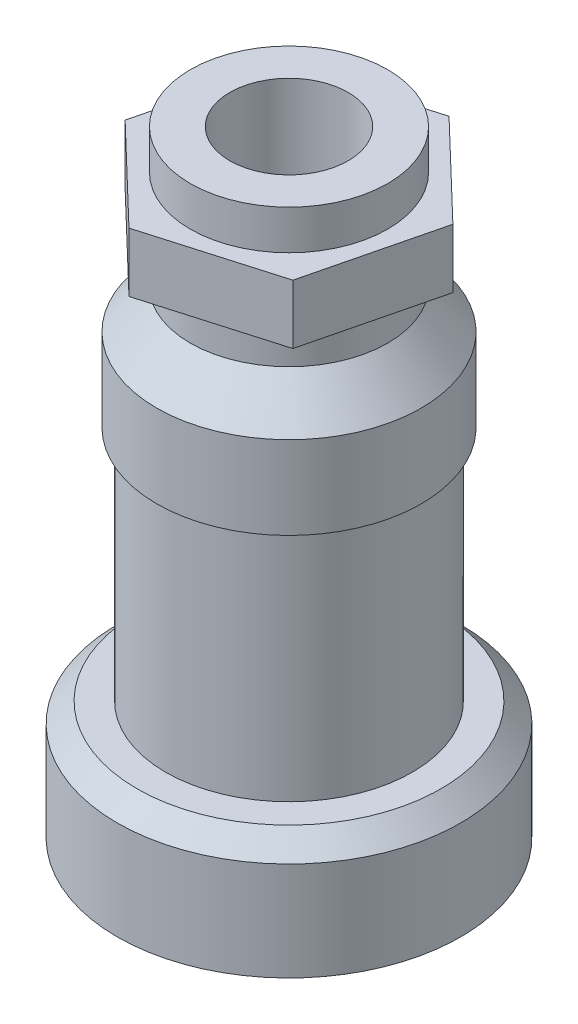
SolidWorks part; units mm, degrees
ref_plane "Front Plane" through (0, 0, 0) normal (0, 0, 1) x (1, 0, 0)
ref_plane "Top Plane" through (0, 0, 0) normal (0, 1, 0) x (1, 0, 0)
ref_plane "Right Plane" through (0, 0, 0) normal (1, 0, 0) x (0, 0, -1)
sketch "Sketch1" plane through (0, 0, 0) normal (0, 0, 1) x (1, 0, 0)
  line L0 (0, 0) -> (0, -35.4245) construction
  line L1 (0, 0) -> (5, 0)
  line L2 (5, 0) -> (5, -7)
  line L4 (5, -7) -> (6.7, -9)
  line L5 (6.7, -9) -> (6.7, -13.2)
  line L6 (6.7, -13.2) -> (6.25, -13.2)
  line L7 (6.25, -13.2) -> (6.25, -25.2)
  line L8 (6.25, -25.2) -> (8.7, -25.2)
  line L9 (8.7, -25.2) -> (8.7, -31.2)
  line L10 (8.7, -31.2) -> (0, -31.2)
  line L11 (0, -31.2) -> (0, 0)
  dimension "D1" = 5
  dimension "D2" = 7
  dimension "D3" = 6.7
  dimension "D4" = 2
  dimension "D5" = 4.2
  dimension "D6" = 6.25
  dimension "D7" = 12
  dimension "D8" = 8.7
  dimension "D9" = 6
revolve "Revolve1" add sketch "Sketch1" angle 360 about L0
ref_plane "Plane1" through (0, -2, 0) normal (0, 1, 0) x (1, 0, 0)
sketch "Sketch2" plane through (0, -2, 0) normal (0, 1, 0) x (1, 0, 0)
  line L1 (-1.6001, -6.5061) -> (4.8344, -4.6388)
  line L2 (4.8344, -4.6388) -> (6.4345, 1.8674)
  line L3 (6.4345, 1.8674) -> (1.6001, 6.5061)
  line L4 (1.6001, 6.5061) -> (-4.8344, 4.6388)
  line L5 (-4.8344, 4.6388) -> (-6.4345, -1.8674)
  line L6 (-6.4345, -1.8674) -> (-1.6001, -6.5061)
  circle A0 centre (0, 0) radius 5.8024 construction
extrude "Boss-Extrude1" add sketch "Sketch2" against normal blind 3
sketch "Sketch3" plane through (0, 0, 0) normal (0, 1, 0) x (1, 0, 0)
  circle A0 centre (0, 0) radius 3
  dimension "D1" = 6
extrude "Cut-Extrude1" cut sketch "Sketch3" against normal through all
chamfer "Chamfer1" distance 1 angle 45 1 edges at (0, -25.2, 8.7)
